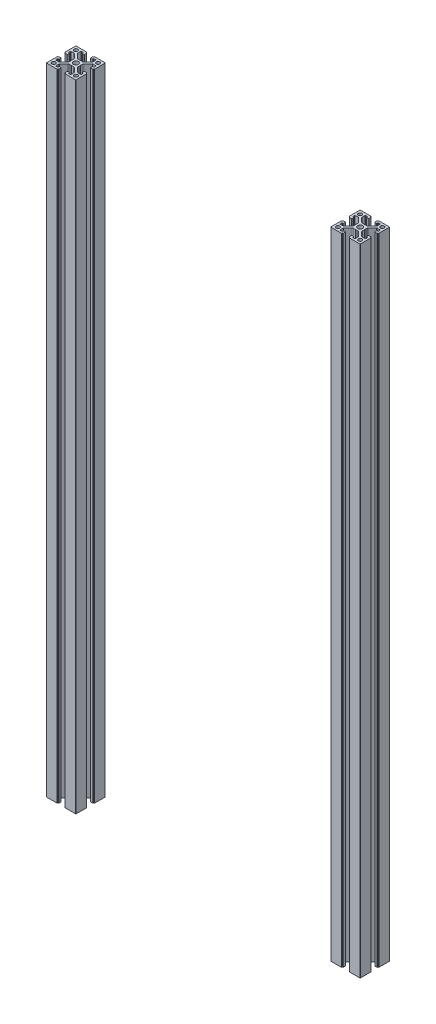
from build123d import *

# Parameters (mm, degrees)
SKETCH_14_R                = 2.45
SKETCH_14_R_2              = 3.4
LE_8_5050W_DEPTH           = 861
SKETCH_14_ON_SEGMENT_2_R   = 2.45
SKETCH_14_ON_SEGMENT_2_R_2 = 3.4
LE_8_5050W_2_DEPTH         = 861


with BuildPart() as part:
    # 草图14 → LE-8-5050W (new body)
    with BuildSketch(Plane(origin=(-192.5, 0, 0), x_dir=(-1, 0, 0), z_dir=(0, 1, 0))):
        with BuildLine():
            Line((-6, -0.3), (-6, -3.050252532))
            ThreePointArc((-6, -3.050252532), (-6.152240935, -3.815619396), (-6.585786438, -4.464466094))
            Line((-6.585786438, -4.464466094), (-12.224873734, -10.103553391))
            ThreePointArc((-12.224873734, -10.103553391), (-12.387085409, -10.211939766), (-12.578427125, -10.25))
            Line((-12.578427125, -10.25), (-16.8, -10.25))
            ThreePointArc((-16.8, -10.25), (-17.153553391, -10.103553391), (-17.3, -9.75))
            Line((-17.3, -9.75), (-17.3, -7.6))
            ThreePointArc((-17.3, -7.6), (-17.153553391, -7.246446609), (-16.8, -7.1))
            Line((-16.8, -7.1), (-16, -7.1))
            ThreePointArc((-16, -7.1), (-15.646446609, -6.953553391), (-15.5, -6.6))
            Line((-15.5, -6.6), (-15.5, -4.6))
            ThreePointArc((-15.5, -4.6), (-15.646446609, -4.246446609), (-16, -4.1))
            Line((-16, -4.1), (-18.7, -4.1))
            ThreePointArc((-18.7, -4.1), (-18.912132034, -4.187867966), (-19, -4.4))
            Line((-19, -4.4), (-19, -4.8))
            ThreePointArc((-19, -4.8), (-19.087867966, -5.012132034), (-19.3, -5.1))
            Line((-19.3, -5.1), (-19.7, -5.1))
            ThreePointArc((-19.7, -5.1), (-19.912132034, -5.187867966), (-20, -5.4))
            Line((-20, -5.4), (-20, -19.5))
            ThreePointArc((-20, -19.5), (-19.853553391, -19.853553391), (-19.5, -20))
            Line((-19.5, -20), (-5.4, -20))
            ThreePointArc((-5.4, -20), (-5.187867966, -19.912132034), (-5.1, -19.7))
            Line((-5.1, -19.7), (-5.1, -19.3))
            ThreePointArc((-5.1, -19.3), (-5.012132034, -19.087867966), (-4.8, -19))
            Line((-4.8, -19), (-4.4, -19))
            ThreePointArc((-4.4, -19), (-4.187867966, -18.912132034), (-4.1, -18.7))
            Line((-4.1, -18.7), (-4.1, -16))
            ThreePointArc((-4.1, -16), (-4.246446609, -15.646446609), (-4.6, -15.5))
            Line((-4.6, -15.5), (-6.6, -15.5))
            ThreePointArc((-6.6, -15.5), (-6.953553391, -15.646446609), (-7.1, -16))
            Line((-7.1, -16), (-7.1, -16.8))
            ThreePointArc((-7.1, -16.8), (-7.246446609, -17.153553391), (-7.6, -17.3))
            Line((-7.6, -17.3), (-9.75, -17.3))
            ThreePointArc((-9.75, -17.3), (-10.103553391, -17.153553391), (-10.25, -16.8))
            Line((-10.25, -16.8), (-10.25, -12.578427125))
            ThreePointArc((-10.25, -12.578427125), (-10.211939766, -12.387085409), (-10.103553391, -12.224873734))
            Line((-10.103553391, -12.224873734), (-4.464466094, -6.585786438))
            ThreePointArc((-4.464466094, -6.585786438), (-3.815619396, -6.152240935), (-3.050252532, -6))
            Line((-3.050252532, -6), (-0.3, -6))
            ThreePointArc((-0.3, -6), (0, -5.7), (0.3, -6))
            Line((0.3, -6), (3.050252532, -6))
            ThreePointArc((3.050252532, -6), (3.815619396, -6.152240935), (4.464466094, -6.585786438))
            Line((4.464466094, -6.585786438), (10.103553391, -12.224873734))
            ThreePointArc((10.103553391, -12.224873734), (10.211939766, -12.387085409), (10.25, -12.578427125))
            Line((10.25, -12.578427125), (10.25, -16.8))
            ThreePointArc((10.25, -16.8), (10.103553391, -17.153553391), (9.75, -17.3))
            Line((9.75, -17.3), (7.6, -17.3))
            ThreePointArc((7.6, -17.3), (7.246446609, -17.153553391), (7.1, -16.8))
            Line((7.1, -16.8), (7.1, -16))
            ThreePointArc((7.1, -16), (6.953553391, -15.646446609), (6.6, -15.5))
            Line((6.6, -15.5), (4.6, -15.5))
            ThreePointArc((4.6, -15.5), (4.246446609, -15.646446609), (4.1, -16))
            Line((4.1, -16), (4.1, -18.7))
            ThreePointArc((4.1, -18.7), (4.187867966, -18.912132034), (4.4, -19))
            Line((4.4, -19), (4.8, -19))
            ThreePointArc((4.8, -19), (5.012132034, -19.087867966), (5.1, -19.3))
            Line((5.1, -19.3), (5.1, -19.7))
            ThreePointArc((5.1, -19.7), (5.187867966, -19.912132034), (5.4, -20))
            Line((5.4, -20), (19.5, -20))
            ThreePointArc((19.5, -20), (19.853553391, -19.853553391), (20, -19.5))
            Line((20, -19.5), (20, -5.4))
            ThreePointArc((20, -5.4), (19.912132034, -5.187867966), (19.7, -5.1))
            Line((19.7, -5.1), (19.3, -5.1))
            ThreePointArc((19.3, -5.1), (19.087867966, -5.012132034), (19, -4.8))
            Line((19, -4.8), (19, -4.4))
            ThreePointArc((19, -4.4), (18.912132034, -4.187867966), (18.7, -4.1))
            Line((18.7, -4.1), (16, -4.1))
            ThreePointArc((16, -4.1), (15.646446609, -4.246446609), (15.5, -4.6))
            Line((15.5, -4.6), (15.5, -6.6))
            ThreePointArc((15.5, -6.6), (15.646446609, -6.953553391), (16, -7.1))
            Line((16, -7.1), (16.8, -7.1))
            ThreePointArc((16.8, -7.1), (17.153553391, -7.246446609), (17.3, -7.6))
            Line((17.3, -7.6), (17.3, -9.75))
            ThreePointArc((17.3, -9.75), (17.153553391, -10.103553391), (16.8, -10.25))
            Line((16.8, -10.25), (12.578427125, -10.25))
            ThreePointArc((12.578427125, -10.25), (12.387085409, -10.211939766), (12.224873734, -10.103553391))
            Line((12.224873734, -10.103553391), (6.585786438, -4.464466094))
            ThreePointArc((6.585786438, -4.464466094), (6.152240935, -3.815619396), (6, -3.050252532))
            Line((6, -3.050252532), (6, -0.3))
            ThreePointArc((6, -0.3), (5.7, 0), (6, 0.3))
            Line((6, 0.3), (6, 3.050252532))
            ThreePointArc((6, 3.050252532), (6.152240935, 3.815619396), (6.585786438, 4.464466094))
            Line((6.585786438, 4.464466094), (12.224873734, 10.103553391))
            ThreePointArc((12.224873734, 10.103553391), (12.387085409, 10.211939766), (12.578427125, 10.25))
            Line((12.578427125, 10.25), (16.8, 10.25))
            ThreePointArc((16.8, 10.25), (17.153553391, 10.103553391), (17.3, 9.75))
            Line((17.3, 9.75), (17.3, 7.6))
            ThreePointArc((17.3, 7.6), (17.153553391, 7.246446609), (16.8, 7.1))
            Line((16.8, 7.1), (16, 7.1))
            ThreePointArc((16, 7.1), (15.646446609, 6.953553391), (15.5, 6.6))
            Line((15.5, 6.6), (15.5, 4.6))
            ThreePointArc((15.5, 4.6), (15.646446609, 4.246446609), (16, 4.1))
            Line((16, 4.1), (18.7, 4.1))
            ThreePointArc((18.7, 4.1), (18.912132034, 4.187867966), (19, 4.4))
            Line((19, 4.4), (19, 4.8))
            ThreePointArc((19, 4.8), (19.087867966, 5.012132034), (19.3, 5.1))
            Line((19.3, 5.1), (19.7, 5.1))
            ThreePointArc((19.7, 5.1), (19.912132034, 5.187867966), (20, 5.4))
            Line((20, 5.4), (20, 19.5))
            ThreePointArc((20, 19.5), (19.853553391, 19.853553391), (19.5, 20))
            Line((19.5, 20), (5.4, 20))
            ThreePointArc((5.4, 20), (5.187867966, 19.912132034), (5.1, 19.7))
            Line((5.1, 19.7), (5.1, 19.3))
            ThreePointArc((5.1, 19.3), (5.012132034, 19.087867966), (4.8, 19))
            Line((4.8, 19), (4.4, 19))
            ThreePointArc((4.4, 19), (4.187867966, 18.912132034), (4.1, 18.7))
            Line((4.1, 18.7), (4.1, 16))
            ThreePointArc((4.1, 16), (4.246446609, 15.646446609), (4.6, 15.5))
            Line((4.6, 15.5), (6.6, 15.5))
            ThreePointArc((6.6, 15.5), (6.953553391, 15.646446609), (7.1, 16))
            Line((7.1, 16), (7.1, 16.8))
            ThreePointArc((7.1, 16.8), (7.246446609, 17.153553391), (7.6, 17.3))
            Line((7.6, 17.3), (9.75, 17.3))
            ThreePointArc((9.75, 17.3), (10.103553391, 17.153553391), (10.25, 16.8))
            Line((10.25, 16.8), (10.25, 12.578427125))
            ThreePointArc((10.25, 12.578427125), (10.211939766, 12.387085409), (10.103553391, 12.224873734))
            Line((10.103553391, 12.224873734), (4.464466094, 6.585786438))
            ThreePointArc((4.464466094, 6.585786438), (3.815619396, 6.152240935), (3.050252532, 6))
            Line((3.050252532, 6), (0.3, 6))
            ThreePointArc((0.3, 6), (0, 5.7), (-0.3, 6))
            Line((-0.3, 6), (-3.050252532, 6))
            ThreePointArc((-3.050252532, 6), (-3.815619396, 6.152240935), (-4.464466094, 6.585786438))
            Line((-4.464466094, 6.585786438), (-10.103553391, 12.224873734))
            ThreePointArc((-10.103553391, 12.224873734), (-10.211939766, 12.387085409), (-10.25, 12.578427125))
            Line((-10.25, 12.578427125), (-10.25, 16.8))
            ThreePointArc((-10.25, 16.8), (-10.103553391, 17.153553391), (-9.75, 17.3))
            Line((-9.75, 17.3), (-7.6, 17.3))
            ThreePointArc((-7.6, 17.3), (-7.246446609, 17.153553391), (-7.1, 16.8))
            Line((-7.1, 16.8), (-7.1, 16))
            ThreePointArc((-7.1, 16), (-6.953553391, 15.646446609), (-6.6, 15.5))
            Line((-6.6, 15.5), (-4.6, 15.5))
            ThreePointArc((-4.6, 15.5), (-4.246446609, 15.646446609), (-4.1, 16))
            Line((-4.1, 16), (-4.1, 18.7))
            ThreePointArc((-4.1, 18.7), (-4.187867966, 18.912132034), (-4.4, 19))
            Line((-4.4, 19), (-4.8, 19))
            ThreePointArc((-4.8, 19), (-5.012132034, 19.087867966), (-5.1, 19.3))
            Line((-5.1, 19.3), (-5.1, 19.7))
            ThreePointArc((-5.1, 19.7), (-5.187867966, 19.912132034), (-5.4, 20))
            Line((-5.4, 20), (-19.5, 20))
            ThreePointArc((-19.5, 20), (-19.853553391, 19.853553391), (-20, 19.5))
            Line((-20, 19.5), (-20, 5.4))
            ThreePointArc((-20, 5.4), (-19.912132034, 5.187867966), (-19.7, 5.1))
            Line((-19.7, 5.1), (-19.3, 5.1))
            ThreePointArc((-19.3, 5.1), (-19.087867966, 5.012132034), (-19, 4.8))
            Line((-19, 4.8), (-19, 4.4))
            ThreePointArc((-19, 4.4), (-18.912132034, 4.187867966), (-18.7, 4.1))
            Line((-18.7, 4.1), (-16, 4.1))
            ThreePointArc((-16, 4.1), (-15.646446609, 4.246446609), (-15.5, 4.6))
            Line((-15.5, 4.6), (-15.5, 6.6))
            ThreePointArc((-15.5, 6.6), (-15.646446609, 6.953553391), (-16, 7.1))
            Line((-16, 7.1), (-16.8, 7.1))
            ThreePointArc((-16.8, 7.1), (-17.153553391, 7.246446609), (-17.3, 7.6))
            Line((-17.3, 7.6), (-17.3, 9.75))
            ThreePointArc((-17.3, 9.75), (-17.153553391, 10.103553391), (-16.8, 10.25))
            Line((-16.8, 10.25), (-12.578427125, 10.25))
            ThreePointArc((-12.578427125, 10.25), (-12.387085409, 10.211939766), (-12.224873734, 10.103553391))
            Line((-12.224873734, 10.103553391), (-6.585786438, 4.464466094))
            ThreePointArc((-6.585786438, 4.464466094), (-6.152240935, 3.815619396), (-6, 3.050252532))
            Line((-6, 3.050252532), (-6, 0.3))
            ThreePointArc((-6, 0.3), (-5.7, 0), (-6, -0.3))
        make_face()
        with Locations((-15, 15)):
            Circle(SKETCH_14_R, mode=Mode.SUBTRACT)
        Circle(SKETCH_14_R_2, mode=Mode.SUBTRACT)
        with Locations((15, 15)):
            Circle(SKETCH_14_R, mode=Mode.SUBTRACT)
        with Locations((15, -15)):
            Circle(SKETCH_14_R, mode=Mode.SUBTRACT)
        with Locations((-15, -15)):
            Circle(SKETCH_14_R, mode=Mode.SUBTRACT)
    extrude(amount=LE_8_5050W_DEPTH)


with BuildPart() as body_2:
    # 草图14 on segment 2 (carried to segment 2) → LE-8-5050W 2 (new body)
    with BuildSketch(Plane(origin=(192.5, 0, 0), x_dir=(-1, 0, 0), z_dir=(0, 1, 0))):
        with BuildLine():
            Line((-6, -0.3), (-6, -3.050252532))
            ThreePointArc((-6, -3.050252532), (-6.152240935, -3.815619396), (-6.585786438, -4.464466094))
            Line((-6.585786438, -4.464466094), (-12.224873734, -10.103553391))
            ThreePointArc((-12.224873734, -10.103553391), (-12.387085409, -10.211939766), (-12.578427125, -10.25))
            Line((-12.578427125, -10.25), (-16.8, -10.25))
            ThreePointArc((-16.8, -10.25), (-17.153553391, -10.103553391), (-17.3, -9.75))
            Line((-17.3, -9.75), (-17.3, -7.6))
            ThreePointArc((-17.3, -7.6), (-17.153553391, -7.246446609), (-16.8, -7.1))
            Line((-16.8, -7.1), (-16, -7.1))
            ThreePointArc((-16, -7.1), (-15.646446609, -6.953553391), (-15.5, -6.6))
            Line((-15.5, -6.6), (-15.5, -4.6))
            ThreePointArc((-15.5, -4.6), (-15.646446609, -4.246446609), (-16, -4.1))
            Line((-16, -4.1), (-18.7, -4.1))
            ThreePointArc((-18.7, -4.1), (-18.912132034, -4.187867966), (-19, -4.4))
            Line((-19, -4.4), (-19, -4.8))
            ThreePointArc((-19, -4.8), (-19.087867966, -5.012132034), (-19.3, -5.1))
            Line((-19.3, -5.1), (-19.7, -5.1))
            ThreePointArc((-19.7, -5.1), (-19.912132034, -5.187867966), (-20, -5.4))
            Line((-20, -5.4), (-20, -19.5))
            ThreePointArc((-20, -19.5), (-19.853553391, -19.853553391), (-19.5, -20))
            Line((-19.5, -20), (-5.4, -20))
            ThreePointArc((-5.4, -20), (-5.187867966, -19.912132034), (-5.1, -19.7))
            Line((-5.1, -19.7), (-5.1, -19.3))
            ThreePointArc((-5.1, -19.3), (-5.012132034, -19.087867966), (-4.8, -19))
            Line((-4.8, -19), (-4.4, -19))
            ThreePointArc((-4.4, -19), (-4.187867966, -18.912132034), (-4.1, -18.7))
            Line((-4.1, -18.7), (-4.1, -16))
            ThreePointArc((-4.1, -16), (-4.246446609, -15.646446609), (-4.6, -15.5))
            Line((-4.6, -15.5), (-6.6, -15.5))
            ThreePointArc((-6.6, -15.5), (-6.953553391, -15.646446609), (-7.1, -16))
            Line((-7.1, -16), (-7.1, -16.8))
            ThreePointArc((-7.1, -16.8), (-7.246446609, -17.153553391), (-7.6, -17.3))
            Line((-7.6, -17.3), (-9.75, -17.3))
            ThreePointArc((-9.75, -17.3), (-10.103553391, -17.153553391), (-10.25, -16.8))
            Line((-10.25, -16.8), (-10.25, -12.578427125))
            ThreePointArc((-10.25, -12.578427125), (-10.211939766, -12.387085409), (-10.103553391, -12.224873734))
            Line((-10.103553391, -12.224873734), (-4.464466094, -6.585786438))
            ThreePointArc((-4.464466094, -6.585786438), (-3.815619396, -6.152240935), (-3.050252532, -6))
            Line((-3.050252532, -6), (-0.3, -6))
            ThreePointArc((-0.3, -6), (0, -5.7), (0.3, -6))
            Line((0.3, -6), (3.050252532, -6))
            ThreePointArc((3.050252532, -6), (3.815619396, -6.152240935), (4.464466094, -6.585786438))
            Line((4.464466094, -6.585786438), (10.103553391, -12.224873734))
            ThreePointArc((10.103553391, -12.224873734), (10.211939766, -12.387085409), (10.25, -12.578427125))
            Line((10.25, -12.578427125), (10.25, -16.8))
            ThreePointArc((10.25, -16.8), (10.103553391, -17.153553391), (9.75, -17.3))
            Line((9.75, -17.3), (7.6, -17.3))
            ThreePointArc((7.6, -17.3), (7.246446609, -17.153553391), (7.1, -16.8))
            Line((7.1, -16.8), (7.1, -16))
            ThreePointArc((7.1, -16), (6.953553391, -15.646446609), (6.6, -15.5))
            Line((6.6, -15.5), (4.6, -15.5))
            ThreePointArc((4.6, -15.5), (4.246446609, -15.646446609), (4.1, -16))
            Line((4.1, -16), (4.1, -18.7))
            ThreePointArc((4.1, -18.7), (4.187867966, -18.912132034), (4.4, -19))
            Line((4.4, -19), (4.8, -19))
            ThreePointArc((4.8, -19), (5.012132034, -19.087867966), (5.1, -19.3))
            Line((5.1, -19.3), (5.1, -19.7))
            ThreePointArc((5.1, -19.7), (5.187867966, -19.912132034), (5.4, -20))
            Line((5.4, -20), (19.5, -20))
            ThreePointArc((19.5, -20), (19.853553391, -19.853553391), (20, -19.5))
            Line((20, -19.5), (20, -5.4))
            ThreePointArc((20, -5.4), (19.912132034, -5.187867966), (19.7, -5.1))
            Line((19.7, -5.1), (19.3, -5.1))
            ThreePointArc((19.3, -5.1), (19.087867966, -5.012132034), (19, -4.8))
            Line((19, -4.8), (19, -4.4))
            ThreePointArc((19, -4.4), (18.912132034, -4.187867966), (18.7, -4.1))
            Line((18.7, -4.1), (16, -4.1))
            ThreePointArc((16, -4.1), (15.646446609, -4.246446609), (15.5, -4.6))
            Line((15.5, -4.6), (15.5, -6.6))
            ThreePointArc((15.5, -6.6), (15.646446609, -6.953553391), (16, -7.1))
            Line((16, -7.1), (16.8, -7.1))
            ThreePointArc((16.8, -7.1), (17.153553391, -7.246446609), (17.3, -7.6))
            Line((17.3, -7.6), (17.3, -9.75))
            ThreePointArc((17.3, -9.75), (17.153553391, -10.103553391), (16.8, -10.25))
            Line((16.8, -10.25), (12.578427125, -10.25))
            ThreePointArc((12.578427125, -10.25), (12.387085409, -10.211939766), (12.224873734, -10.103553391))
            Line((12.224873734, -10.103553391), (6.585786438, -4.464466094))
            ThreePointArc((6.585786438, -4.464466094), (6.152240935, -3.815619396), (6, -3.050252532))
            Line((6, -3.050252532), (6, -0.3))
            ThreePointArc((6, -0.3), (5.7, 0), (6, 0.3))
            Line((6, 0.3), (6, 3.050252532))
            ThreePointArc((6, 3.050252532), (6.152240935, 3.815619396), (6.585786438, 4.464466094))
            Line((6.585786438, 4.464466094), (12.224873734, 10.103553391))
            ThreePointArc((12.224873734, 10.103553391), (12.387085409, 10.211939766), (12.578427125, 10.25))
            Line((12.578427125, 10.25), (16.8, 10.25))
            ThreePointArc((16.8, 10.25), (17.153553391, 10.103553391), (17.3, 9.75))
            Line((17.3, 9.75), (17.3, 7.6))
            ThreePointArc((17.3, 7.6), (17.153553391, 7.246446609), (16.8, 7.1))
            Line((16.8, 7.1), (16, 7.1))
            ThreePointArc((16, 7.1), (15.646446609, 6.953553391), (15.5, 6.6))
            Line((15.5, 6.6), (15.5, 4.6))
            ThreePointArc((15.5, 4.6), (15.646446609, 4.246446609), (16, 4.1))
            Line((16, 4.1), (18.7, 4.1))
            ThreePointArc((18.7, 4.1), (18.912132034, 4.187867966), (19, 4.4))
            Line((19, 4.4), (19, 4.8))
            ThreePointArc((19, 4.8), (19.087867966, 5.012132034), (19.3, 5.1))
            Line((19.3, 5.1), (19.7, 5.1))
            ThreePointArc((19.7, 5.1), (19.912132034, 5.187867966), (20, 5.4))
            Line((20, 5.4), (20, 19.5))
            ThreePointArc((20, 19.5), (19.853553391, 19.853553391), (19.5, 20))
            Line((19.5, 20), (5.4, 20))
            ThreePointArc((5.4, 20), (5.187867966, 19.912132034), (5.1, 19.7))
            Line((5.1, 19.7), (5.1, 19.3))
            ThreePointArc((5.1, 19.3), (5.012132034, 19.087867966), (4.8, 19))
            Line((4.8, 19), (4.4, 19))
            ThreePointArc((4.4, 19), (4.187867966, 18.912132034), (4.1, 18.7))
            Line((4.1, 18.7), (4.1, 16))
            ThreePointArc((4.1, 16), (4.246446609, 15.646446609), (4.6, 15.5))
            Line((4.6, 15.5), (6.6, 15.5))
            ThreePointArc((6.6, 15.5), (6.953553391, 15.646446609), (7.1, 16))
            Line((7.1, 16), (7.1, 16.8))
            ThreePointArc((7.1, 16.8), (7.246446609, 17.153553391), (7.6, 17.3))
            Line((7.6, 17.3), (9.75, 17.3))
            ThreePointArc((9.75, 17.3), (10.103553391, 17.153553391), (10.25, 16.8))
            Line((10.25, 16.8), (10.25, 12.578427125))
            ThreePointArc((10.25, 12.578427125), (10.211939766, 12.387085409), (10.103553391, 12.224873734))
            Line((10.103553391, 12.224873734), (4.464466094, 6.585786438))
            ThreePointArc((4.464466094, 6.585786438), (3.815619396, 6.152240935), (3.050252532, 6))
            Line((3.050252532, 6), (0.3, 6))
            ThreePointArc((0.3, 6), (0, 5.7), (-0.3, 6))
            Line((-0.3, 6), (-3.050252532, 6))
            ThreePointArc((-3.050252532, 6), (-3.815619396, 6.152240935), (-4.464466094, 6.585786438))
            Line((-4.464466094, 6.585786438), (-10.103553391, 12.224873734))
            ThreePointArc((-10.103553391, 12.224873734), (-10.211939766, 12.387085409), (-10.25, 12.578427125))
            Line((-10.25, 12.578427125), (-10.25, 16.8))
            ThreePointArc((-10.25, 16.8), (-10.103553391, 17.153553391), (-9.75, 17.3))
            Line((-9.75, 17.3), (-7.6, 17.3))
            ThreePointArc((-7.6, 17.3), (-7.246446609, 17.153553391), (-7.1, 16.8))
            Line((-7.1, 16.8), (-7.1, 16))
            ThreePointArc((-7.1, 16), (-6.953553391, 15.646446609), (-6.6, 15.5))
            Line((-6.6, 15.5), (-4.6, 15.5))
            ThreePointArc((-4.6, 15.5), (-4.246446609, 15.646446609), (-4.1, 16))
            Line((-4.1, 16), (-4.1, 18.7))
            ThreePointArc((-4.1, 18.7), (-4.187867966, 18.912132034), (-4.4, 19))
            Line((-4.4, 19), (-4.8, 19))
            ThreePointArc((-4.8, 19), (-5.012132034, 19.087867966), (-5.1, 19.3))
            Line((-5.1, 19.3), (-5.1, 19.7))
            ThreePointArc((-5.1, 19.7), (-5.187867966, 19.912132034), (-5.4, 20))
            Line((-5.4, 20), (-19.5, 20))
            ThreePointArc((-19.5, 20), (-19.853553391, 19.853553391), (-20, 19.5))
            Line((-20, 19.5), (-20, 5.4))
            ThreePointArc((-20, 5.4), (-19.912132034, 5.187867966), (-19.7, 5.1))
            Line((-19.7, 5.1), (-19.3, 5.1))
            ThreePointArc((-19.3, 5.1), (-19.087867966, 5.012132034), (-19, 4.8))
            Line((-19, 4.8), (-19, 4.4))
            ThreePointArc((-19, 4.4), (-18.912132034, 4.187867966), (-18.7, 4.1))
            Line((-18.7, 4.1), (-16, 4.1))
            ThreePointArc((-16, 4.1), (-15.646446609, 4.246446609), (-15.5, 4.6))
            Line((-15.5, 4.6), (-15.5, 6.6))
            ThreePointArc((-15.5, 6.6), (-15.646446609, 6.953553391), (-16, 7.1))
            Line((-16, 7.1), (-16.8, 7.1))
            ThreePointArc((-16.8, 7.1), (-17.153553391, 7.246446609), (-17.3, 7.6))
            Line((-17.3, 7.6), (-17.3, 9.75))
            ThreePointArc((-17.3, 9.75), (-17.153553391, 10.103553391), (-16.8, 10.25))
            Line((-16.8, 10.25), (-12.578427125, 10.25))
            ThreePointArc((-12.578427125, 10.25), (-12.387085409, 10.211939766), (-12.224873734, 10.103553391))
            Line((-12.224873734, 10.103553391), (-6.585786438, 4.464466094))
            ThreePointArc((-6.585786438, 4.464466094), (-6.152240935, 3.815619396), (-6, 3.050252532))
            Line((-6, 3.050252532), (-6, 0.3))
            ThreePointArc((-6, 0.3), (-5.7, 0), (-6, -0.3))
        make_face()
        with Locations((-15, 15)):
            Circle(SKETCH_14_ON_SEGMENT_2_R, mode=Mode.SUBTRACT)
        Circle(SKETCH_14_ON_SEGMENT_2_R_2, mode=Mode.SUBTRACT)
        with Locations((15, 15)):
            Circle(SKETCH_14_ON_SEGMENT_2_R, mode=Mode.SUBTRACT)
        with Locations((15, -15)):
            Circle(SKETCH_14_ON_SEGMENT_2_R, mode=Mode.SUBTRACT)
        with Locations((-15, -15)):
            Circle(SKETCH_14_ON_SEGMENT_2_R, mode=Mode.SUBTRACT)
    extrude(amount=LE_8_5050W_2_DEPTH)


solid = Compound([part.part, body_2.part])
